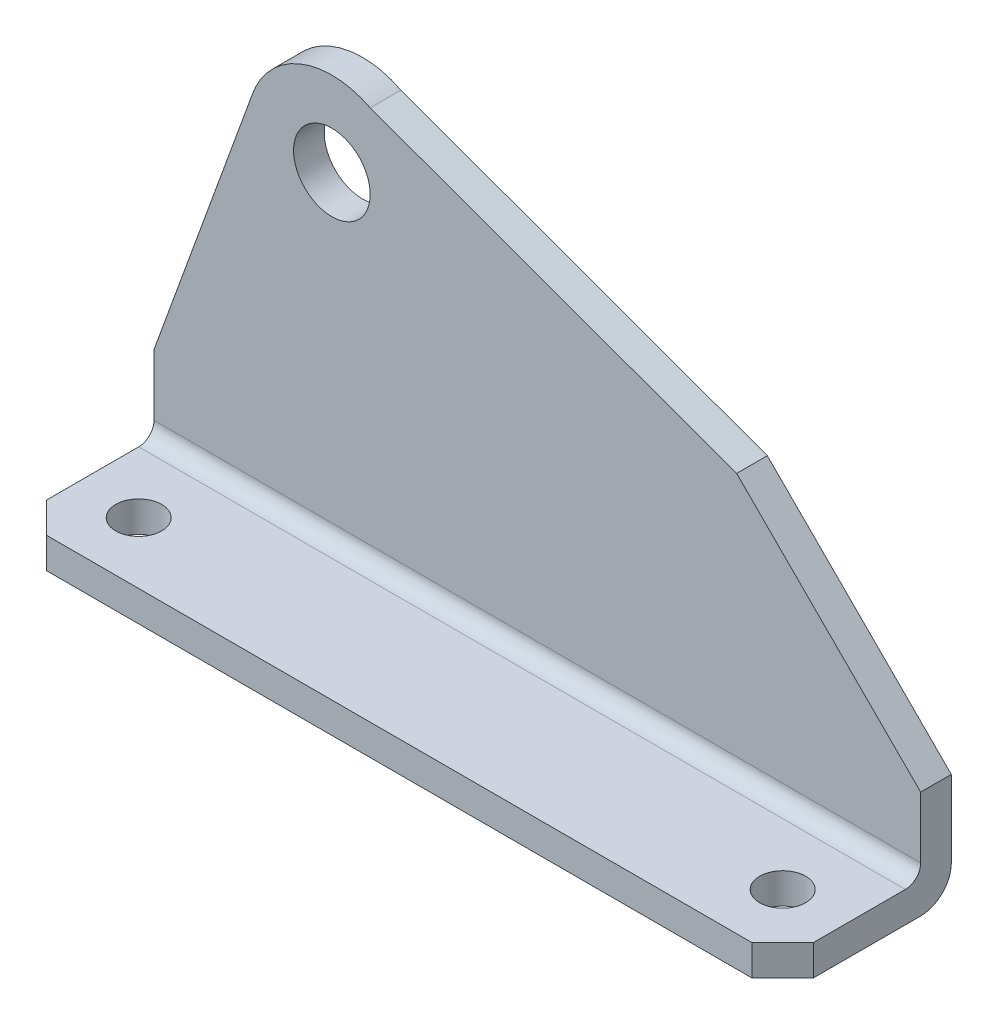
SolidWorks part; units mm, degrees
material "1023 碳钢板 (SS)"
ref_plane "Front Plane" through (0, 0, 0) normal (0, 0, 1) x (1, 0, 0)
ref_plane "Top Plane" through (0, 0, 0) normal (0, 1, 0) x (1, 0, 0)
ref_plane "Right Plane" through (0, 0, 0) normal (1, 0, 0) x (0, 0, -1)
sketch "Sketch1" plane through (0, 0, 0) normal (0, 0, 1) x (1, 0, 0)
  line L1 (125, 90.5) -> (-125, 90.5)
  line L2 (125, 90.5) -> (125, -90.5)
  line L3 (125, -90.5) -> (-125, -90.5)
  line L4 (-125, 90.5) -> (-125, -90.5)
  line L5 (125, 90.5) -> (-125, -90.5) construction
  line L6 (125, -90.5) -> (-125, 90.5) construction
  point P0 (0, 0)
  dimension "D1" = 250
  dimension "D2" = 181
extrude "Boss-Extrude1" add sketch "Sketch1" along normal blind 10 contours L2 L1 L4 L3
sketch "Sketch2" plane through (0, 0, 10) normal (0, 0, 1) x (1, 0, 0)
  line L0 (-125, -55.5) -> (-93.1599, 31.98)
  line L1 (-125, 90.5) -> (-125, -90.5) construction
  line L2 (125, -90.5) -> (-125, -90.5) construction
  line L3 (125, -55.5) -> (65, 4.5)
  line L4 (125, 90.5) -> (125, -90.5) construction
  line L5 (65, 4.5) -> (-54.4969, 47.9933)
  line L6 (-125, -55.5) -> (-125, -90.5)
  line L7 (-125, -90.5) -> (125, -90.5)
  line L8 (125, -90.5) -> (125, -55.5)
  arc A0 (-54.4969, 47.9933) -> (-93.1599, 31.98) centre (-67, 23.5) ccw
  dimension "D4" = 55
  dimension "D5" = 58
  dimension "D1" = 35
  dimension "D2" = 70
  dimension "D3" = 114
  dimension "D6" = 35
  dimension "D7" = 60
  dimension "D8" = 60
  dimension "D9" = 90
extrude "Cut-Extrude1" cut sketch "Sketch2" against normal blind 10 flip side to cut
sketch "Sketch3" plane through (0, 0, 10) normal (0, 0, 1) x (1, 0, 0)
  line L0 (125, -90.5) -> (-125, -90.5) construction
  line L1 (-125, -55.5) -> (-125, -90.5) construction
  circle A0 centre (-67, 23.5) radius 12.5
  dimension "D1" = 25
  dimension "D3" = 58
  dimension "D2" = 114
extrude "Cut-Extrude2" cut sketch "Sketch3" against normal blind 10
sketch "Sketch6" plane through (0, 0, 10) normal (0, 0, 1) x (1, 0, 0)
  line L0 (-125, -80.5) -> (125, -80.5)
  line L1 (-125, -55.5) -> (-125, -90.5) construction
  line L2 (125, -55.5) -> (125, -90.5) construction
  line L3 (125, -80.5) -> (125, -90.5)
  line L4 (125, -90.5) -> (-125, -90.5)
  line L5 (-125, -90.5) -> (-125, -80.5)
  dimension "D1" = 10
extrude "Boss-Extrude3" add sketch "Sketch6" along normal blind 45
fillet "Fillet3" radius 5 1 edges at (0, -80.5, 10)
fillet "Fillet4" radius 10 1 edges at (0, -90.5, 0)
sketch "Sketch7" plane through (0, -90.5, 0) normal (0, -1, 0) x (1, 0, 0)
  line L0 (125, 0) -> (-125, 0) construction
  line L1 (-125, 55) -> (-125, 10) construction
  circle A0 centre (-105, 35) radius 7.5
  circle A1 centre (105, 35) radius 7.5
  dimension "D2" = 35
  dimension "D3" = 20
  dimension "D4" = 15
  dimension "D1" = 210
extrude "Cut-Extrude4" cut sketch "Sketch7" against normal blind 45
chamfer "Chamfer2" distance 10 angle 45 2 edges at (125, -85.5, 55) (-125, -85.5, 55)
